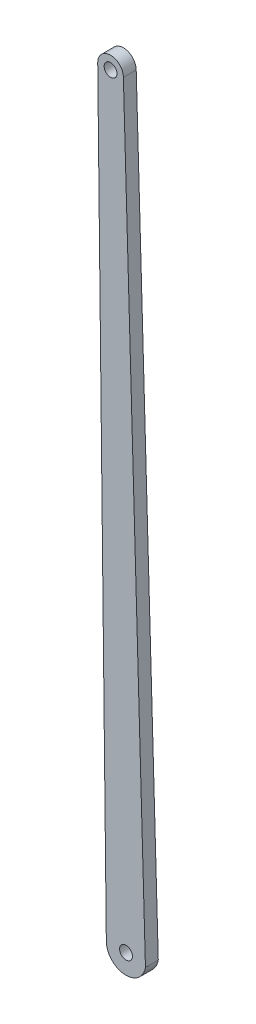
SolidWorks part; units mm, degrees
ref_plane "Front Plane" through (0, 0, 0) normal (0, 0, 1) x (1, 0, 0)
ref_plane "Top Plane" through (0, 0, 0) normal (0, 1, 0) x (1, 0, 0)
ref_plane "Right Plane" through (0, 0, 0) normal (1, 0, 0) x (0, 0, -1)
other "Configuration Table"
sketch "Sketch3" plane through (0, 0, 0) normal (0, 0, 1) x (1, 0, 0)
  line L0 (0.1864, 1267.7117) -> (0.2083, 1277.7117) construction
  line L1 (-3.0142, 681.3639) -> (27.5, 684.5414) construction
  line L2 (-15, 796.4658) -> (70, -19.8021) construction
  line L3 (10.1973, 1272.7117) -> (27.3948, 680.5604)
  line L4 (100, -16.6782) -> (15, 799.5897) construction
  line L5 (-3.0957, 682.7783) -> (-9.8027, 1272.7117)
  arc A0 (25.8478, 1256.0979) -> (-25.5255, 1256.2102) centre (0.1114, 1233.389) ccw construction
  arc A1 (33.3461, 1262.7142) -> (-32.9948, 1262.8592) centre (0.1114, 1233.389) ccw construction
  circle A2 centre (0.1973, 1272.7117) radius 5
  arc A3 (10.1973, 1272.7117) -> (-9.8001, 1272.4844) centre (0.1973, 1272.7117) ccw
  arc A4 (-3.0957, 682.7783) -> (27.2304, 686.2202) centre (12.2429, 682.9526) ccw
  circle A5 centre (12.2429, 682.9526) radius 5
  arc M5 (25.8478, 1256.0979) -> (-25.5255, 1256.2102) centre (0.1114, 1233.389) ccw
  arc M7 (-32.9948, 1262.8592) -> (33.3461, 1262.7142) centre (0.1114, 1233.389) cw
  arc M10 (-19.4017, 1179.6138) -> (19.3758, 1179.501) centre (0, 1184) ccw
  circle M16 centre (0, 1184) radius 5
extrude "Boss-Extrude1" add sketch "Sketch3" along normal blind 10 contours L5 A4 L3 A5 M10 | L5 L3 M10 M5 M16 | L3 A3 A2 M7 M5 | A3 M7 | A3 L5 A2 M7 M5 | M16
